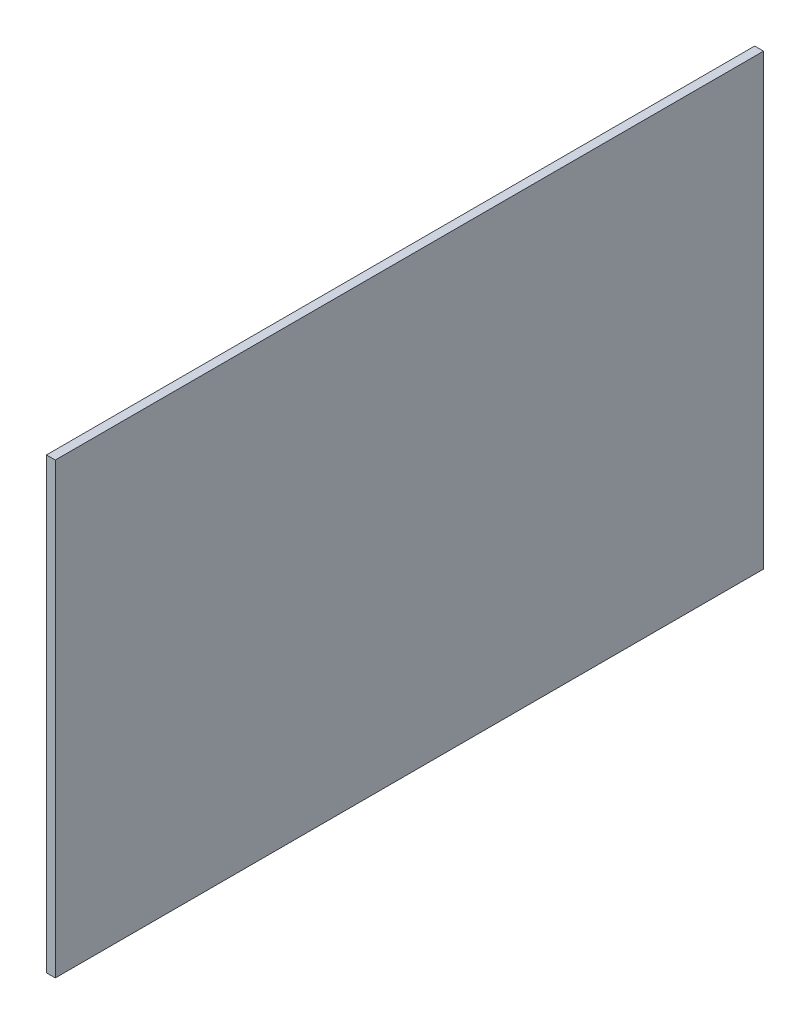
from build123d import *

# Parameters (mm, degrees)
SKETCH_1_W           = 120
SKETCH_1_H           = 76
BOSS_EXTRUDE_1_DEPTH = 1.5


with BuildPart() as part:
    # Sketch 1 → Boss-Extrude 1 (new body)
    with BuildSketch(Plane(origin=(0, 0, 0), x_dir=(0, 0, -1), z_dir=(1, 0, 0))):
        Rectangle(SKETCH_1_W, SKETCH_1_H)
    extrude(amount=BOSS_EXTRUDE_1_DEPTH)


solid = part.part
